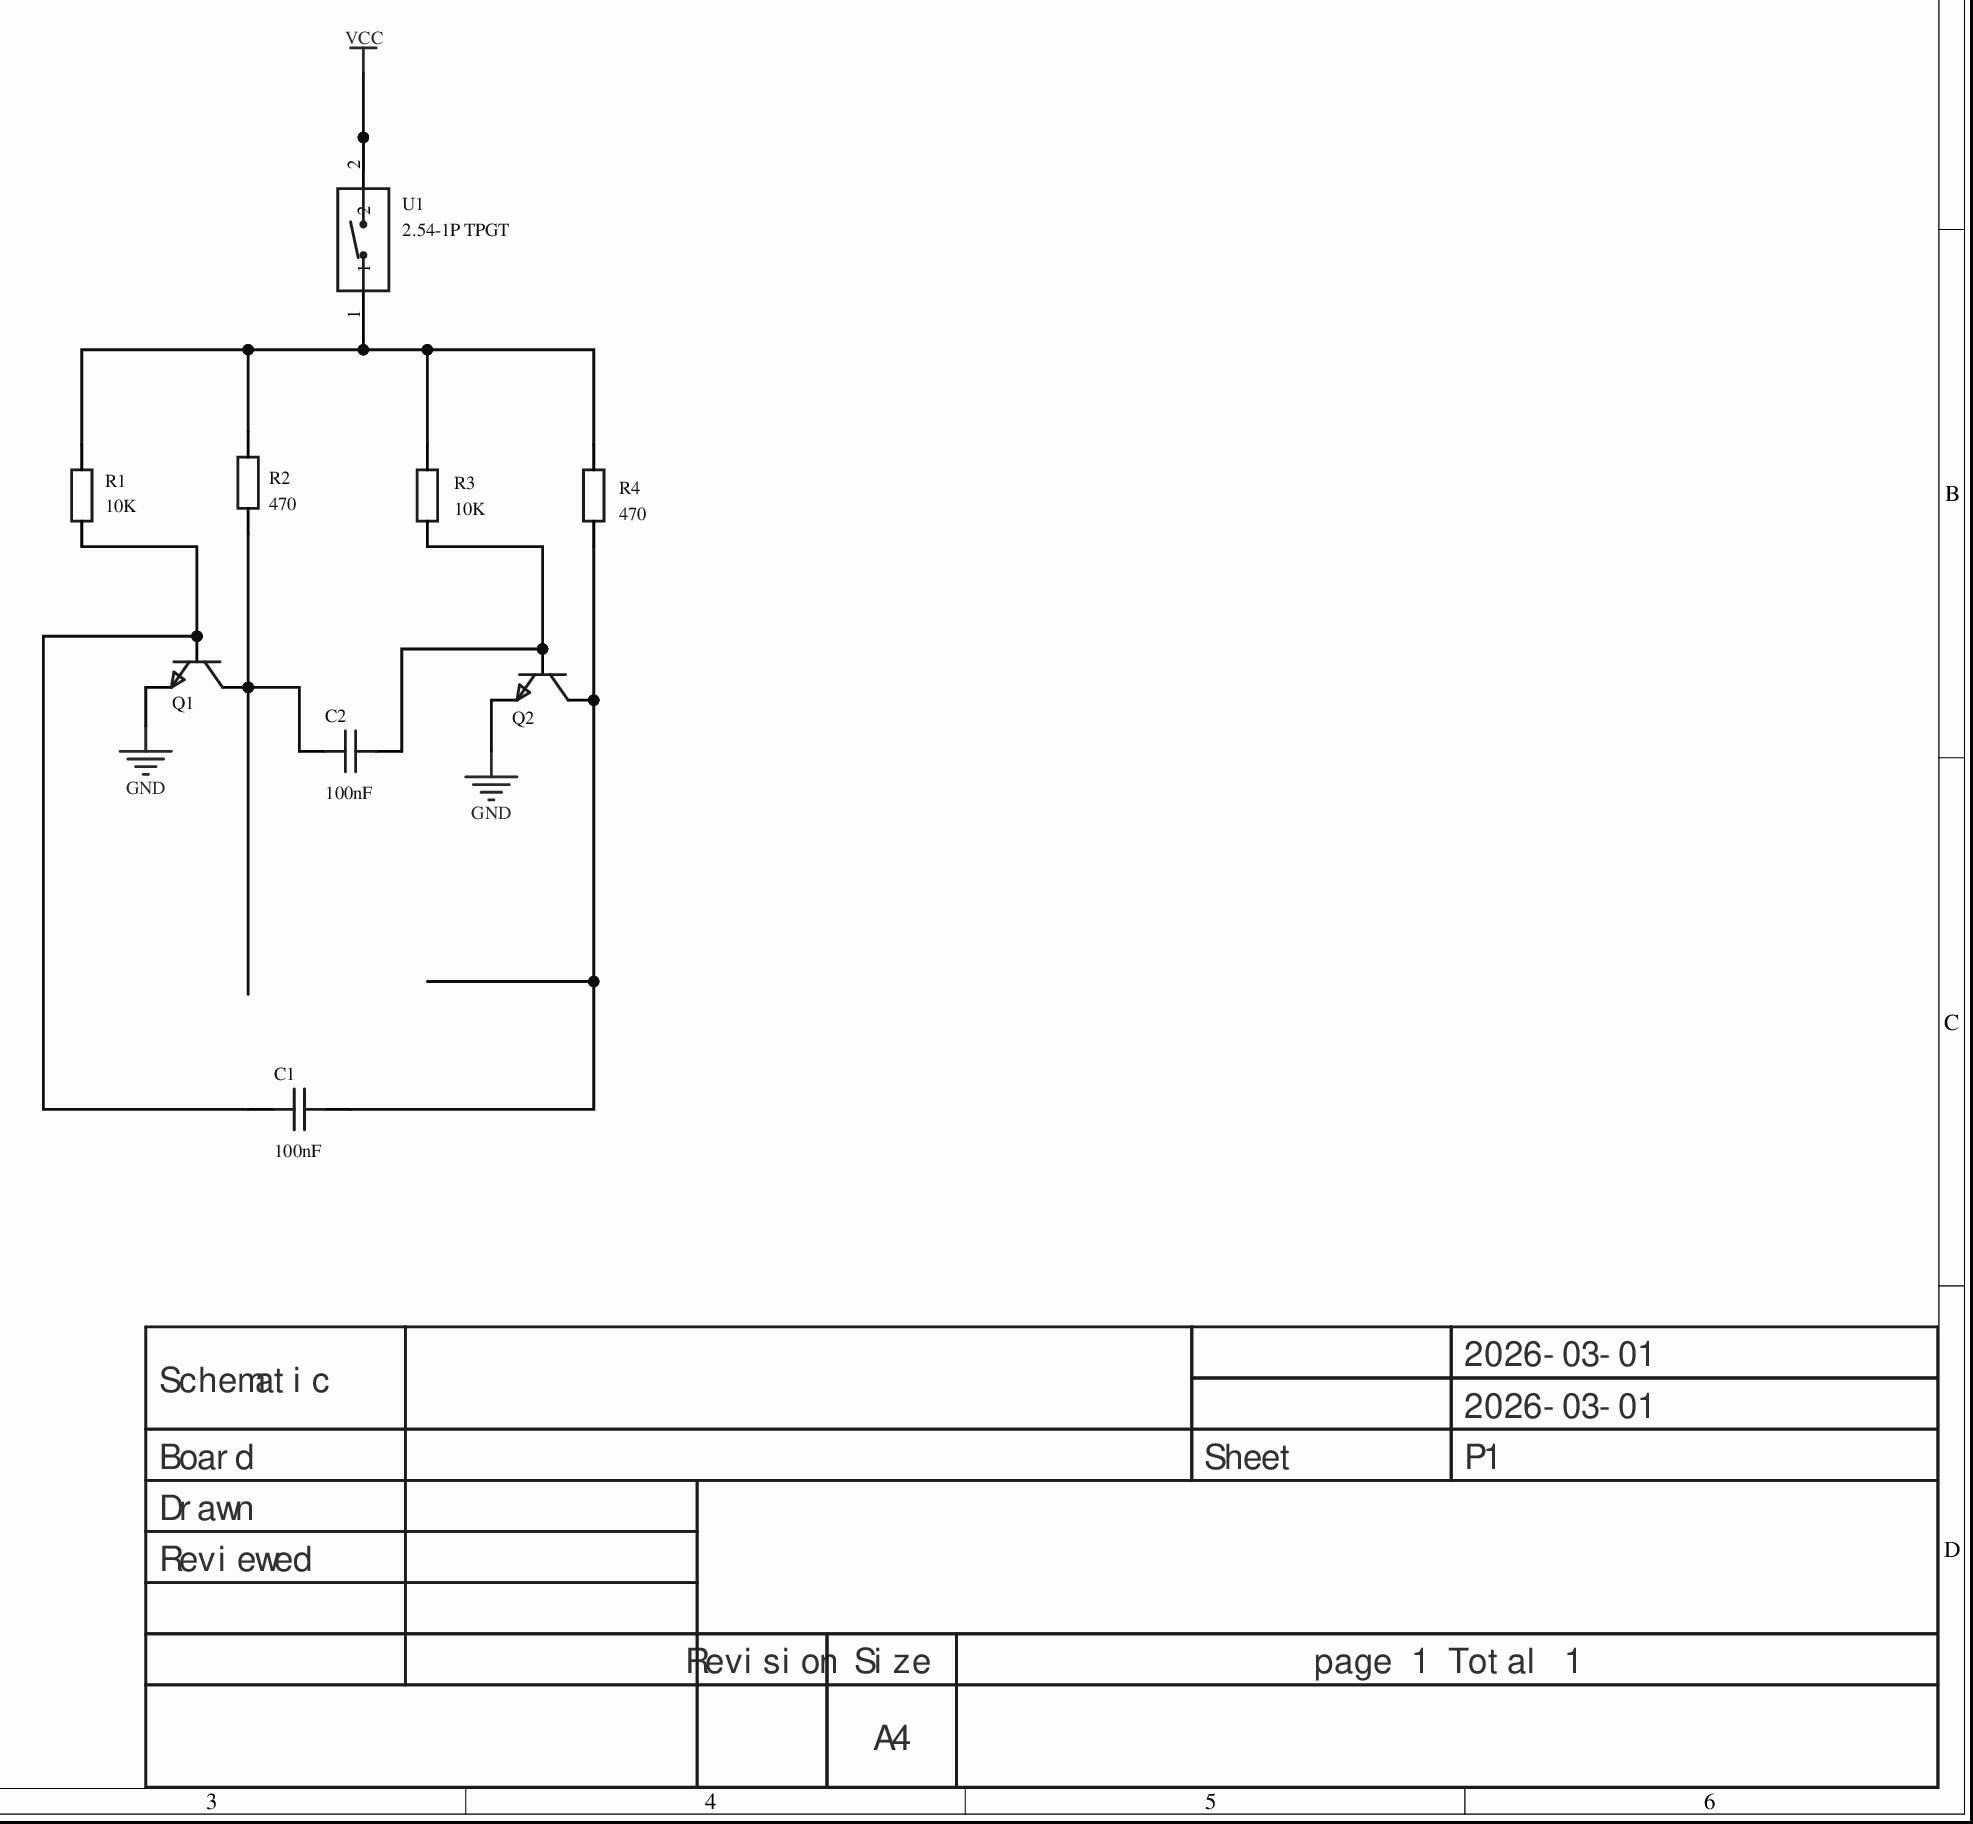
[diagram p0: MISC52073-3.schdoc]
# Altium project MISC52073-2.PrjPcb
1 sheet, 9 parts. Net scope: global (net labels, ports and power ports of the same name join across sheets).
Board file: MISC52073.pcbdoc

## Sheet MISC52073-3.schdoc
size 297 x 209 mm; Version: V1.0; @Project Name: MISC52073; @Update Date: 2026-03-01; @Create Date: 2026-03-01; @Board Name: MISC52073; @Create Time: 19:19:06; @Page Count: 1; @Page No: 1; @Schematic Name: MISC52073; @Update Time: 19:19:06; Size: A4

### Parts
C1  100nF  [C0603]
C2  100nF  [C0603]
Q1  (no value)  [S8050_SOT-23]
Q2  (no value)  [S8050_SOT-23]
R1  10K  [R0603]
R2  470  [R0603]
R3  10K  [R0603]
R4  470  [R0603]
U1  2.54-1P TPGT  [SW-SMD_2P-L6.2-W2.5-LS9.4]

### Nets
GND: Q1.2 Q2.2
VCC: U1.2
NetC1_1: C1.1 Q2.3 R4.1
NetC1_2: C1.2 Q1.1 R1.1
NetC2_1: C2.1 Q2.1 R3.1
NetC2_2: C2.2 Q1.3 R2.1
NetR1_2: R1.2 R2.2 R3.2 R4.2 U1.1

### Notes on the sheet
- 2026-03-01
- Schematic
- Board
- Sheet
- P1
- Drawn
- Reviewed
- Revision
- Size
- A4
- page 1 Total 1

### Library data of the parts
C1 C2 = CAP_0603: Symbol: Capacitance; ConvertToPcb: yes; ModelId: ac125912035d415993ca9572d50418b10819f05c4eef4c71ace90d822a990e87; ModelName: C0603_L1.6-W0.8-H0.8; ModelTransform: 62.992,31.496,0,0,0,0,0,0,0; Device: CAP_0603; AddInBom: yes; Supplier Footprint: 0603; FootprintName: C0603; Value: 100nF
Q1 Q2 = S8050_SOT_NPN: Symbol: NPN; ConvertToPcb: yes; ModelId: c62791f0466c4ae2a892c056b845b0ca0819f05c4eef4c71ace90d822a990e87; ModelName: SOT-23-3P_L2.9-W1.3-H1.0-LS2.4-P0.95; ModelTransform: 98.6,114.12,41.29,180,0,0,0,0,-3; Device: S8050_SOT_NPN; AddInBom: yes; Supplier Footprint: SOT-23; FootprintName: S8050_SOT-23
R1-R4 = Res_0603: Symbol: Resistor; ConvertToPcb: yes; ModelId: fc143cca1e79419f9cd78b61e9279f080819f05c4eef4c71ace90d822a990e87; ModelTransform: 31.8897,63.7794,0,90,0,0,0,0,0; Device: Res_0603; AddInBom: yes; Supplier Footprint: 0603; FootprintName: R0603; ModelName: R0603
  R1 R3: Value: 10K
  R2 R4: Value: 470
U1 = 2.54-1P TPGT: 类型:平拨,凸起式;电路结构:单刀单掷;开关位数:1位;额定电流:25mA;额定电压:24V;工作寿命:2千次;颜色:黑色;; Manufacturer: SHOU HAN(首韩); AddInBom: yes; ModelId: 6f54f6d4d657465290acdafbbf6e338f0819f05c4eef4c71ace90d822a990e87; ModelTransform: 370.078,98.425,0,0,0,0,0,0,0; Circuit: SPST; Number of Positions: 1 position; Current Rating: 25mA; Voltage Rating: 24V; Operating Life: 2 thousand cycles; Description: Type: flat-actuated, raised; circuit: SPST; positions: 1; rated current: 25mA; rated voltage: 24V; operating life: 2 thousand cycles; color: black;; Symbol: 2.54-1P TPGT; Device: 2.54-1P TPGT; LCSC Part Name: 2.54-1P贴片高推有LOGO编带; SupplierPart: C7421519; ManufacturerPart: 2.54-1P TPGT; Supplier Footprint: SMD,P=2.54mm; JLCPCB Part Class: Extended Part; Datasheet: https://example.com/datasheet/2.54-1P%2520TPGT/8402822.html; Supplier: LCSC; ConvertToPcb: yes; FootprintName: SW-SMD_2P-L6.2-W2.5-LS9.4; ModelName: SW-SMD_2P-L6.2-W2.5-LS9.4; Type: Flat-actuated, raised; Termination Style: Gull-wing; Lead Pitch: 2.54mm; Operating Temperature: -30℃~+85℃; Color: Black